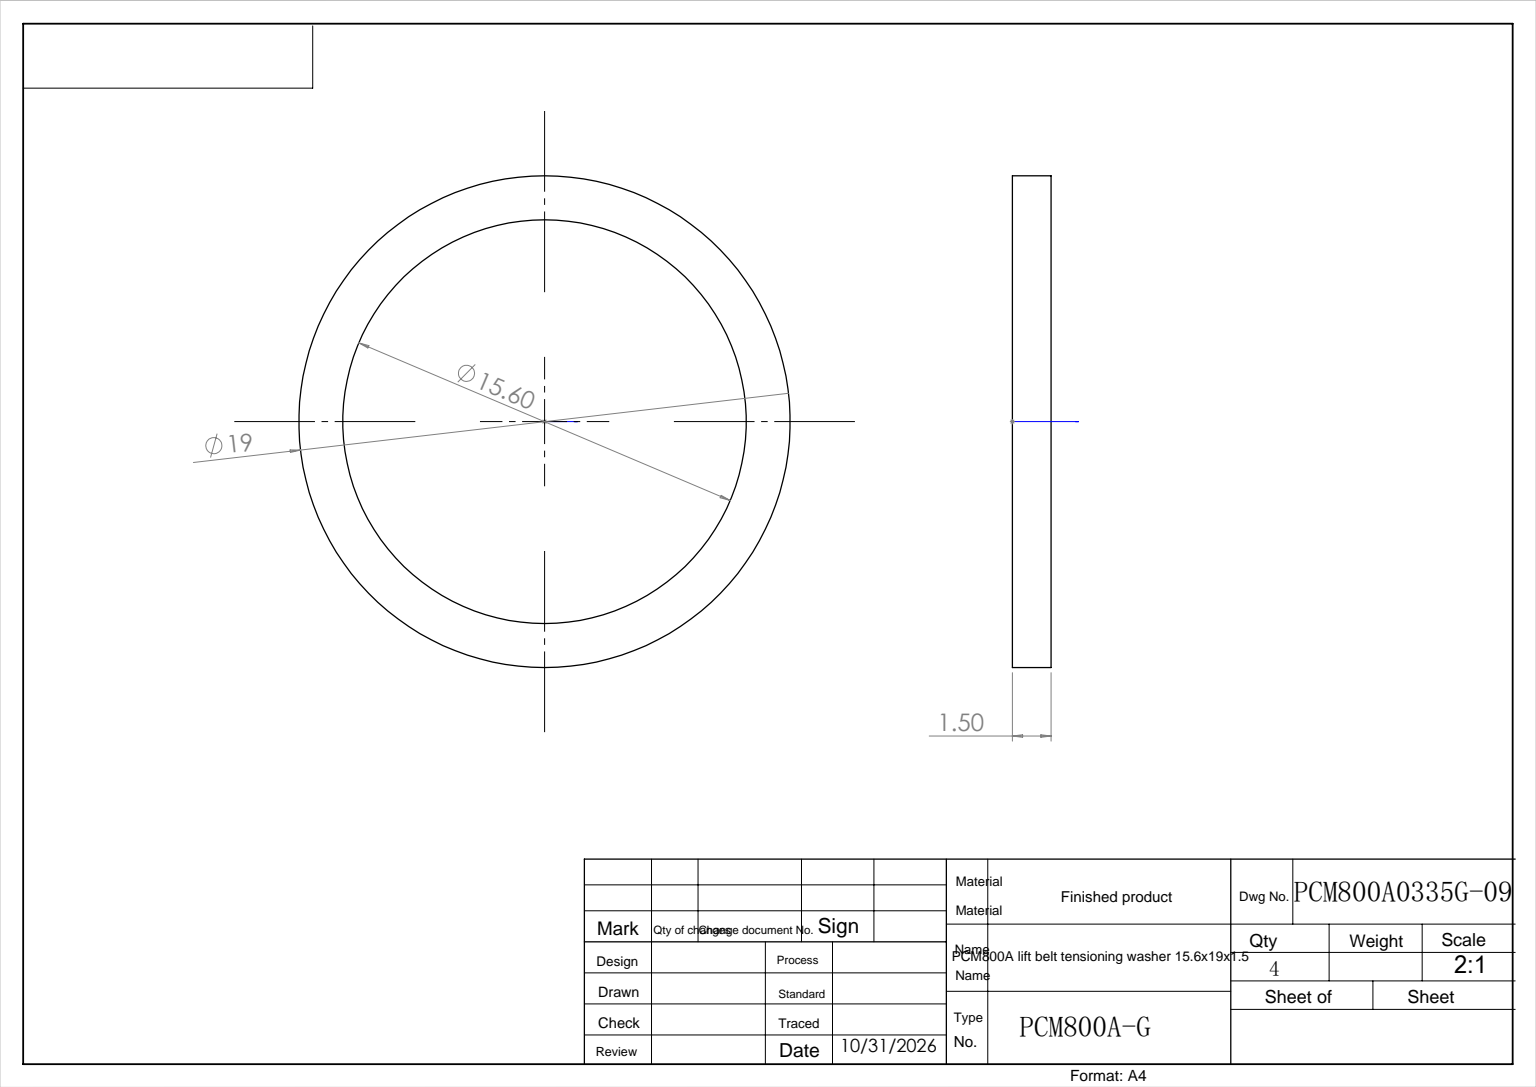
from build123d import *

# Parameters (mm, degrees)
SKETCH_1_R      = 9.5
SKETCH_1_R_2    = 7.8
EXTRUDE_1_DEPTH = 1.5


with BuildPart() as part:
    # 草图1 → 拉伸1 (new body)
    with BuildSketch(Plane(origin=(0, 0, 0), x_dir=(1, 0, 0), z_dir=(0, 1, 0))):
        with Locations(Location((0, 0, 0), (0, 0, 270))):
            Circle(SKETCH_1_R)
        with Locations(Location((0, 0, 0), (0, 0, 270))):
            Circle(SKETCH_1_R_2, mode=Mode.SUBTRACT)
    extrude(amount=EXTRUDE_1_DEPTH)


solid = part.part
